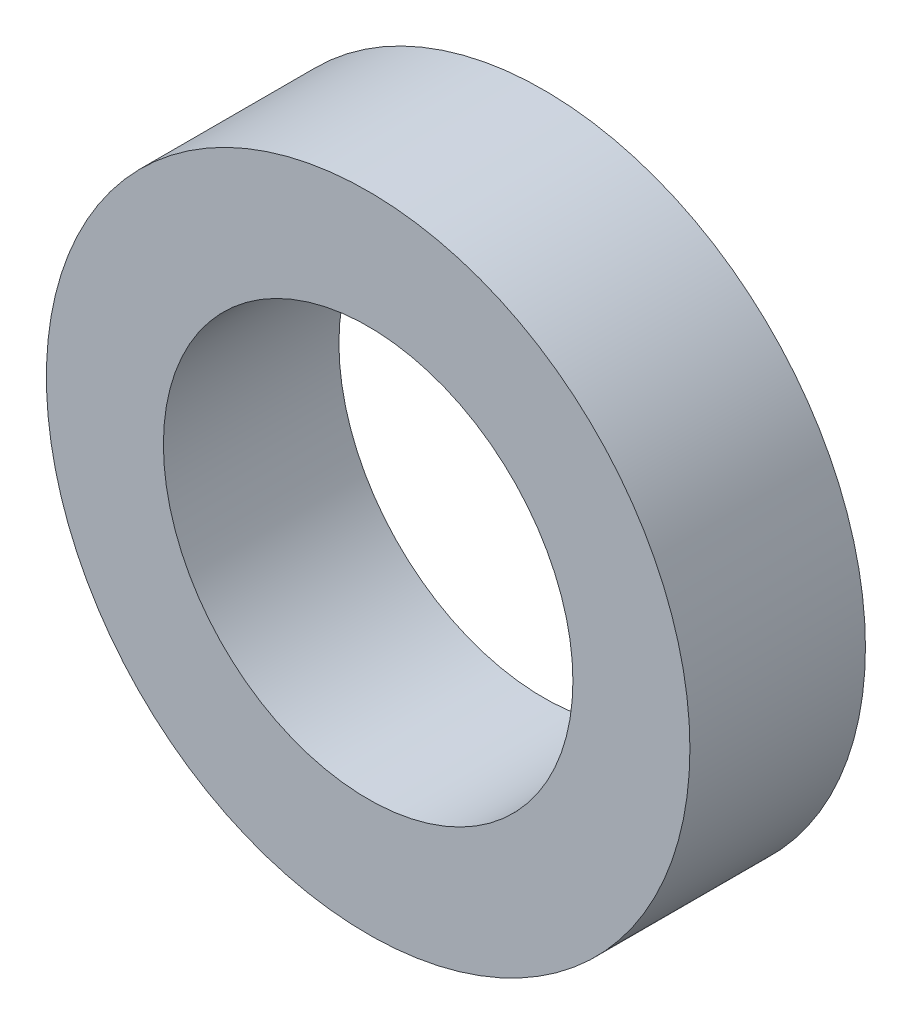
from build123d import *

# Parameters (mm, degrees)
SKETCH1_W = 6
SKETCH1_H = 4


with BuildPart() as part:
    # Sketch1 → Revolve1 (revolve)
    with BuildSketch(Plane(origin=(0, 0, 0), x_dir=(0, 0, -1), z_dir=(1, 0, 0)), mode=Mode.PRIVATE) as revolve1_sk:
        with Locations((3, 9)):
            Rectangle(SKETCH1_W, SKETCH1_H)
    revolve(revolve1_sk.sketch.rotate(Axis((0, 0, 4.548360851), (0, 0, -1)), 90), axis=Axis((0, 0, 4.548360851), (0, 0, -1)))


solid = part.part
